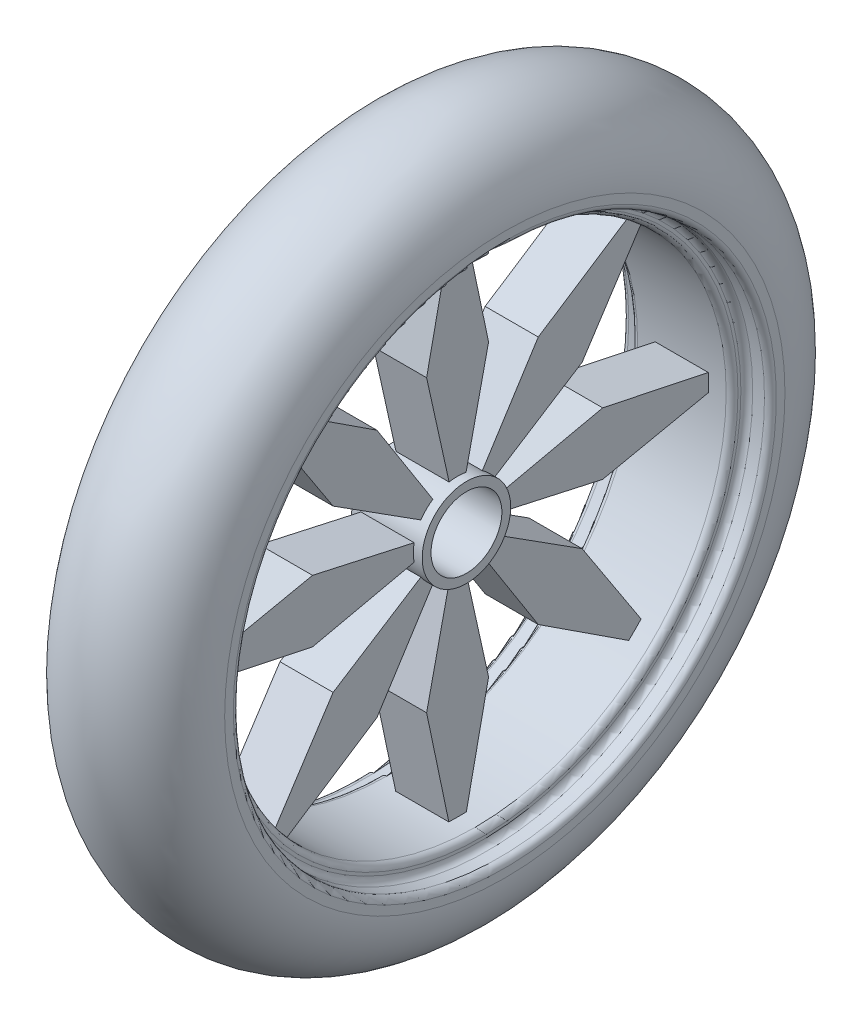
from build123d import *

# Parameters (mm, degrees)
SKETCH2_R           = 90
SKETCH2_R_2         = 85
BOSS_EXTRUDE1_DEPTH = 17
SKETCH3_R           = 15
SKETCH3_R_2         = 12
BOSS_EXTRUDE2_DEPTH = 12
FILLET1_R           = 2
BOSS_EXTRUDE3_DEPTH = 9
CIRPATTERN1_COUNT   = 8


with BuildPart() as part:
    # Sketch1 → Revolve1 (revolve)
    with BuildSketch(Plane.XY, mode=Mode.PRIVATE) as revolve1_sk:
        with BuildLine():
            Line((25, 94.930938799), (25, 90))
            Line((25, 90), (-25, 90))
            Line((-25, 90), (-25, 94.930938799))
            ThreePointArc((-25, 94.930938799), (0, 119.930938799), (25, 94.930938799))
        make_face()
    revolve(revolve1_sk.sketch.rotate(Axis((0, 0, 0), (1, 0, 0)), 90), axis=Axis((0, 0, 0), (1, 0, 0)))

    # Sketch2 → Boss-Extrude1 (add, symmetric)
    with BuildSketch(Plane(origin=(0, 0, 0), x_dir=(0, 0, -1), z_dir=(1, 0, 0))):
        with Locations(Location((0, 0, 0), (0, 0, 180))):
            Circle(SKETCH2_R)
        Circle(SKETCH2_R_2, mode=Mode.SUBTRACT)
    extrude(amount=BOSS_EXTRUDE1_DEPTH, both=True)

    # Fillet1
    fillet1_edges = [part.edges().sort_by_distance(p)[0] for p in [
        (-17, 0, -90),
        (17, 0, -90),
        (-17, 0, 85),
        (17, 0, 85),
        (-25, 0, -90),
        (25, 0, -90),
    ]]
    fillet(fillet1_edges, radius=FILLET1_R)



with BuildPart() as body_2:
    # Sketch3 → Boss-Extrude2 (new, symmetric)
    with BuildSketch(Plane(origin=(0, 0, 0), x_dir=(0, 0, -1), z_dir=(1, 0, 0))):
        with Locations(Location((0, 0, 0), (0, 0, 180))):
            Circle(SKETCH3_R)
        with Locations(Location((0, 0, 0), (0, 0, 180))):
            Circle(SKETCH3_R_2, mode=Mode.SUBTRACT)
    extrude(amount=BOSS_EXTRUDE2_DEPTH, both=True)


with BuildPart() as part_1:
    add(part.part)

    add(body_2.part)  # Boss-Extrude3 merges body 2
    # Sketch4 → Boss-Extrude3 (add, symmetric)
    with BuildSketch(Plane(origin=(0, 0, 0), x_dir=(0, 0, -1), z_dir=(1, 0, 0))):
        Polygon((-2.552768196, 86.962540065), (-10.497348074, 49.156301409), (-2.523426033, 13.169872653), (2.523426033, 13.169872653), (10.497348074, 49.156301409), (2.552768196, 86.962540065), align=None)
    boss_extrude3 = extrude(amount=BOSS_EXTRUDE3_DEPTH, both=True)

    # CirPattern1: Boss-Extrude3 ×8 about axis
    cirpattern1_axis = Axis((0, 0, 0), (1, 0, 0))
    for i in range(1, CIRPATTERN1_COUNT):
        add(boss_extrude3.rotate(cirpattern1_axis, i * 360 / CIRPATTERN1_COUNT))


solid = part_1.part
